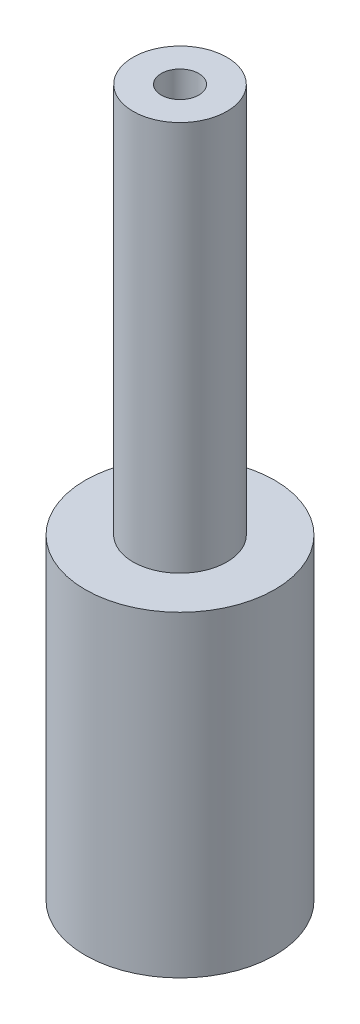
SolidWorks part; units mm, degrees
material "ABS"
ref_plane "Front Plane" through (0, 0, 0) normal (0, 0, 1) x (1, 0, 0)
ref_plane "Top Plane" through (0, 0, 0) normal (0, 1, 0) x (1, 0, 0)
ref_plane "Right Plane" through (0, 0, 0) normal (1, 0, 0) x (0, 0, -1)
sketch "Sketch1" plane through (0, 0, 0) normal (0, 0, 1) x (1, 0, 0)
  line L0 (0, 23.6464) -> (0, 0) construction
  line L1 (-1.25, 8.44) -> (-1.25, 18.84)
  line L2 (-1.25, 8.44) -> (-2.525, 8.44)
  line L3 (-2.525, 0) -> (-2.525, 8.44)
  line L4 (-1.25, 18.84) -> (-0.5, 18.84)
  line L5 (-0.5, 18.84) -> (-0.5, 0)
  line L6 (-0.5, 0) -> (-2.525, 0)
  dimension "D1" = 2.5
  dimension "D2" = 1.275
  dimension "D3" = 1
revolve "Revolve2" add sketch "Sketch1" angle 360 about L0
